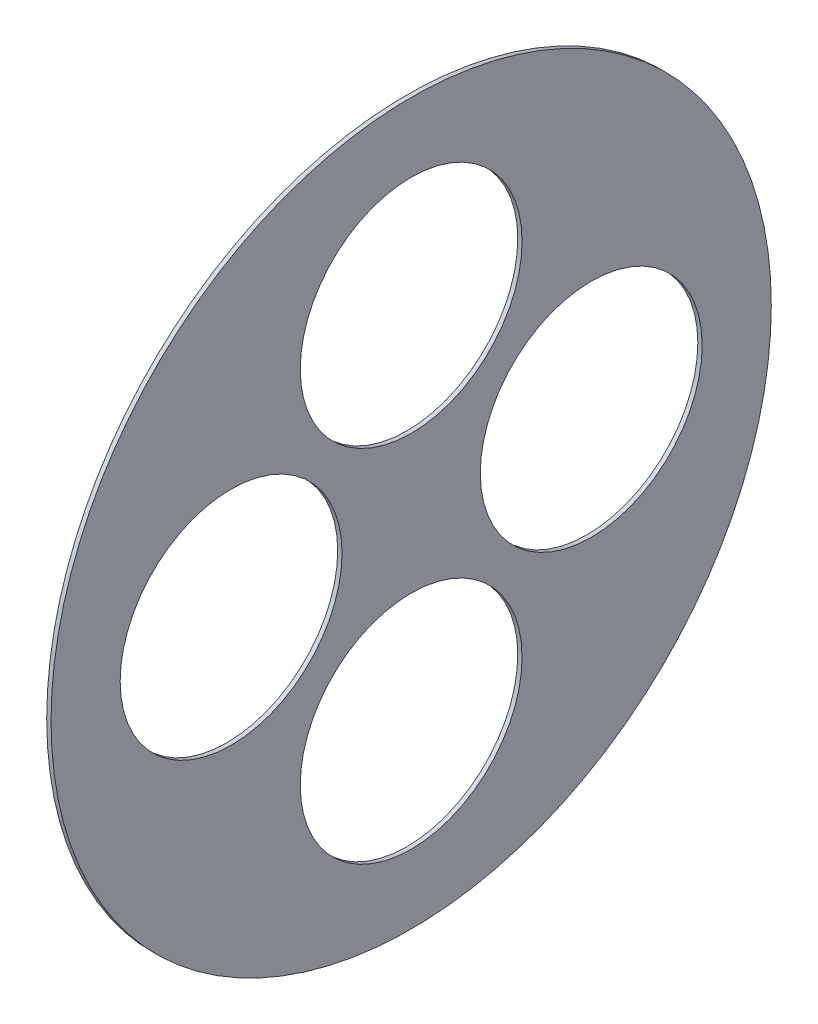
from build123d import *

# Parameters (mm, degrees)
SKETCH1_R           = 250
BOSS_EXTRUDE1_DEPTH = 3
SKETCH2_R           = 77
CUT_EXTRUDE1_DEPTH  = 10
CIRPATTERN1_COUNT   = 4


with BuildPart() as part:
    # Sketch1 → Boss-Extrude1 (new body)
    with BuildSketch(Plane(origin=(0, 0, 0), x_dir=(0, 0, -1), z_dir=(1, 0, 0))):
        Circle(SKETCH1_R)
    extrude(amount=BOSS_EXTRUDE1_DEPTH)

    # Sketch2 → Cut-Extrude1 (cut)
    with BuildSketch(Plane(origin=(3, 0, 0), x_dir=(0, 0, -1), z_dir=(1, 0, 0))):
        with Locations((0, 125)):
            Circle(SKETCH2_R)
    cut_extrude1 = extrude(amount=-CUT_EXTRUDE1_DEPTH, mode=Mode.SUBTRACT)

    # CirPattern1: Cut-Extrude1 ×4 about axis
    cirpattern1_axis = Axis((0, 0, 0), (1, 0, 0))
    for i in range(1, CIRPATTERN1_COUNT):
        add(cut_extrude1.rotate(cirpattern1_axis, i * 360 / CIRPATTERN1_COUNT), mode=Mode.SUBTRACT)


solid = part.part
